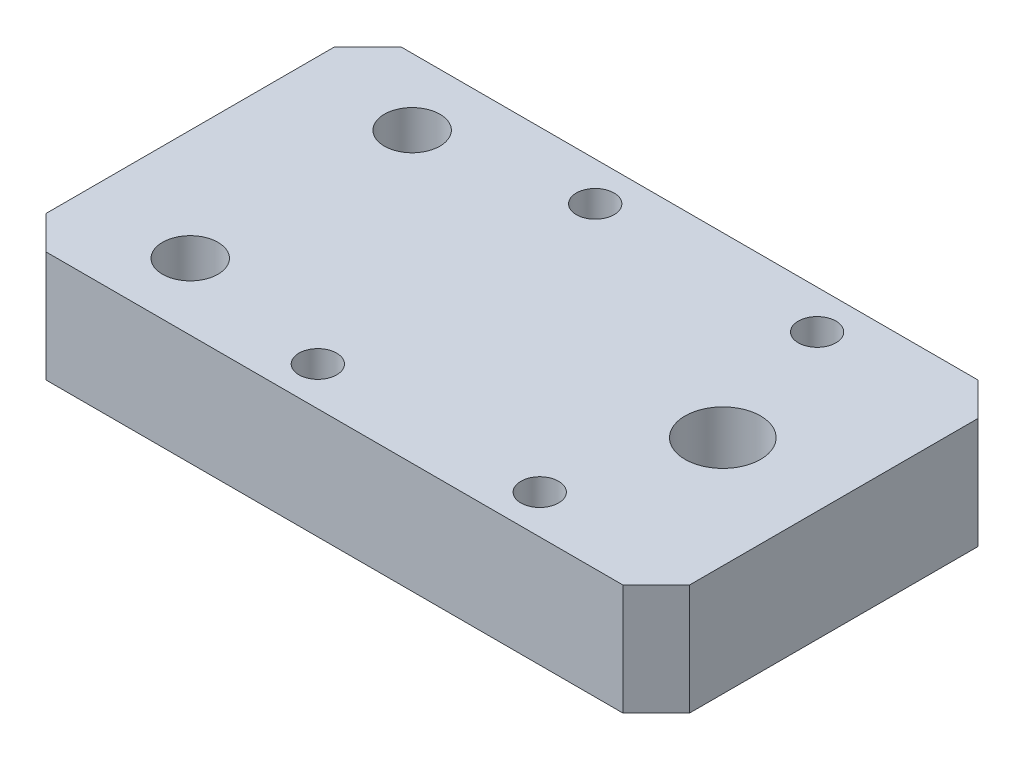
from build123d import *

# Parameters (mm, degrees)
SKETCH1_W                                            = 58
SKETCH1_H                                            = 32
BOSS_EXTRUDE1_DEPTH                                  = 10
CBORE_FOR_M4_HEXAGON_SOCKET_HEAD_CAP_SCR_D           = 3.4
CBORE_FOR_M4_HEXAGON_SOCKET_HEAD_CAP_SCR_DEPTH       = 18.1
CBORE_FOR_M4_HEXAGON_SOCKET_HEAD_CAP_SCR_CBORE_D     = 6
CBORE_FOR_M4_HEXAGON_SOCKET_HEAD_CAP_SCR_CBORE_DEPTH = 3.4
CBORE_FOR_M4_HEXAGON_SOCKET_HEAD_CAP_SCR_TIP         = 1.021463052
M6_TAPPED_HOLE1_D                                    = 5
M6_TAPPED_HOLE1_DEPTH                                = 15
M6_TAPPED_HOLE1_TIP                                  = 1.502151548
M8_TAPPED_HOLE1_D                                    = 6.8
M8_TAPPED_HOLE1_DEPTH                                = 19.75
M8_TAPPED_HOLE1_TIP                                  = 2.042926105
CHAMFER1_SIZE                                        = 3


with BuildPart() as part:
    # Sketch1 → Boss-Extrude1 (new body)
    with BuildSketch(Plane(origin=(0, 0, 0), x_dir=(1, 0, 0), z_dir=(0, 1, 0))):
        Rectangle(SKETCH1_W, SKETCH1_H)
    extrude(amount=BOSS_EXTRUDE1_DEPTH)

    # CBORE for M4 Hexagon socket head cap screws1
    with Locations(Plane(origin=(0, 0, 0), x_dir=(-1, 0, 0), z_dir=(0, -1, 0))):
        with Locations((-15, 12.5), (5, 12.5), (-15, -12.5), (5, -12.5)):
            CounterBoreHole(CBORE_FOR_M4_HEXAGON_SOCKET_HEAD_CAP_SCR_D / 2, CBORE_FOR_M4_HEXAGON_SOCKET_HEAD_CAP_SCR_CBORE_D / 2, CBORE_FOR_M4_HEXAGON_SOCKET_HEAD_CAP_SCR_CBORE_DEPTH, depth=CBORE_FOR_M4_HEXAGON_SOCKET_HEAD_CAP_SCR_DEPTH)
            with Locations((0, 0, -(CBORE_FOR_M4_HEXAGON_SOCKET_HEAD_CAP_SCR_DEPTH + CBORE_FOR_M4_HEXAGON_SOCKET_HEAD_CAP_SCR_TIP / 2))):  # 118° drill point
                Cone(0, CBORE_FOR_M4_HEXAGON_SOCKET_HEAD_CAP_SCR_D / 2, CBORE_FOR_M4_HEXAGON_SOCKET_HEAD_CAP_SCR_TIP, mode=Mode.SUBTRACT)

    # M6 Tapped Hole1
    with Locations(Plane(origin=(0, 0, 0), x_dir=(-1, 0, 0), z_dir=(0, -1, 0))):
        with Locations((19, 10), (19, -10)):
            Hole(M6_TAPPED_HOLE1_D / 2, depth=M6_TAPPED_HOLE1_DEPTH)
            with Locations((0, 0, -(M6_TAPPED_HOLE1_DEPTH + M6_TAPPED_HOLE1_TIP / 2))):  # 118° drill point
                Cone(0, M6_TAPPED_HOLE1_D / 2, M6_TAPPED_HOLE1_TIP, mode=Mode.SUBTRACT)

    # M8 Tapped Hole1
    with Locations(Plane(origin=(0, 0, 0), x_dir=(-1, 0, 0), z_dir=(0, -1, 0))):
        with Locations((-19, 0)):
            Hole(M8_TAPPED_HOLE1_D / 2, depth=M8_TAPPED_HOLE1_DEPTH)
            with Locations((0, 0, -(M8_TAPPED_HOLE1_DEPTH + M8_TAPPED_HOLE1_TIP / 2))):  # 118° drill point
                Cone(0, M8_TAPPED_HOLE1_D / 2, M8_TAPPED_HOLE1_TIP, mode=Mode.SUBTRACT)

    # Chamfer1
    chamfer1_edges = [part.edges().sort_by_distance(p)[0] for p in [
        (29, 5, 16),
        (-29, 5, 16),
        (-29, 5, -16),
        (29, 5, -16),
    ]]
    chamfer(chamfer1_edges, length=CHAMFER1_SIZE)


solid = part.part
